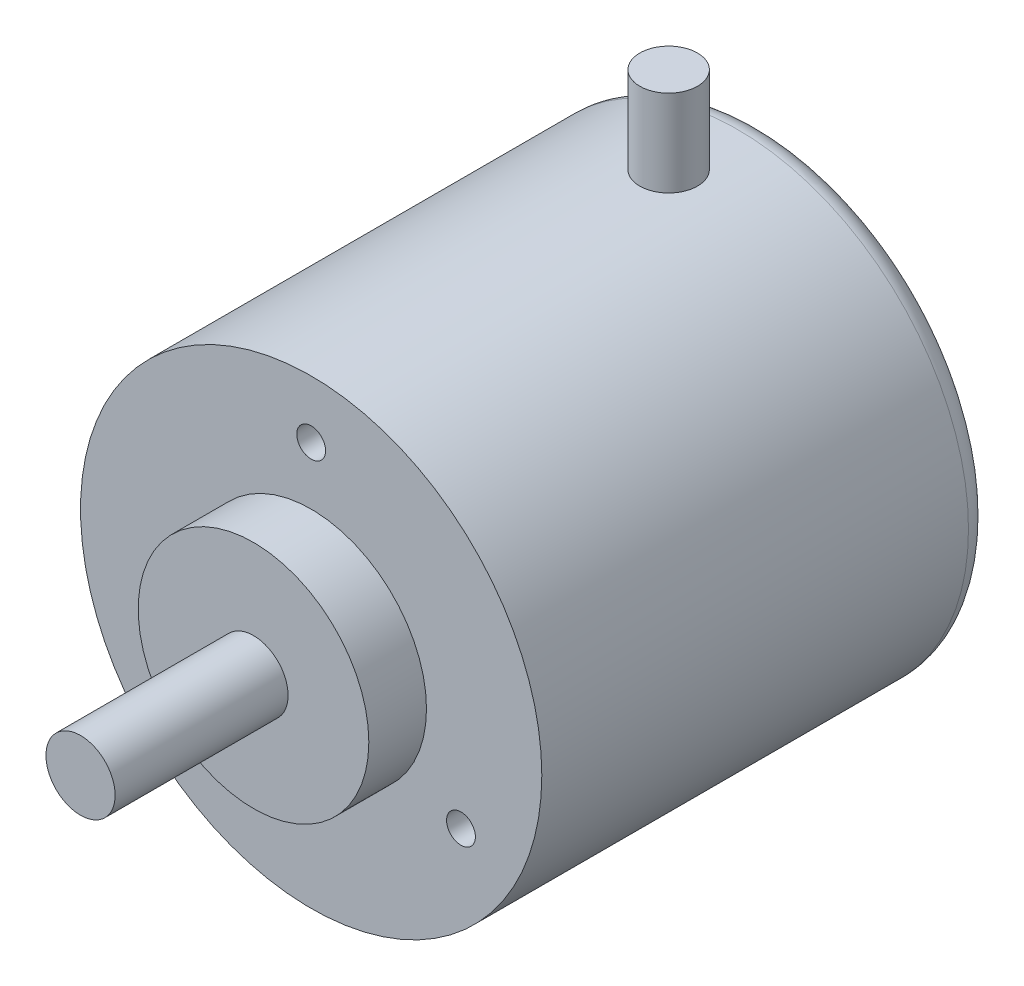
SolidWorks part; units mm, degrees
ref_plane "前视基准面" through (0, 0, 0) normal (0, 0, 1) x (1, 0, 0)
ref_plane "上视基准面" through (0, 0, 0) normal (0, 1, 0) x (1, 0, 0)
ref_plane "右视基准面" through (0, 0, 0) normal (1, 0, 0) x (0, 0, -1)
sketch "草图1" plane through (0, 0, 0) normal (0, 0, 1) x (1, 0, 0)
  circle A0 centre (0, 0) radius 20
extrude "凸台-拉伸1" add sketch "草图1" along normal blind 39
sketch "草图2" plane through (0, 0, 39) normal (0, 0, 1) x (1, 0, 0)
  circle A0 centre (0, 0) radius 10
extrude "凸台-拉伸2" add sketch "草图2" along normal blind 5 separate body
sketch "草图3" plane through (0, 0, 44) normal (0, 0, 1) x (1, 0, 0)
  circle A0 centre (0, 0) radius 3
extrude "凸台-拉伸3" add sketch "草图3" along normal blind 15 separate body
sketch "草图4" plane through (0, 0, 39) normal (0, 0, 1) x (1, 0, 0)
  circle A0 centre (0, 0) radius 15 construction
  circle A1 centre (0, 15) radius 1.5 construction
  circle A2 centre (12.9904, -7.5) radius 1.5 construction
  circle A3 centre (-12.9904, -7.5) radius 1.5 construction
  dimension "D1" = 3
hole_wizard "M3 螺纹孔1" positions "草图5" profile "草图6" tap size "M3" standard "GB"
sketch "草图5" plane through (0, 0, 39) normal (0, 0, 1) x (1, 0, 0)
  circle A0 centre (0, 0) radius 15 construction
  point P0 (0, 15)
  point P4 (-12.9904, -7.5)
  point P7 (12.9904, -7.5)
sketch "草图6" plane through (0, 15, 39) normal (1, 0, 0) x (0, -1, 0)
  line L0 (0, 0) -> (0, 7.5)
  line L1 (0, 7.5) -> (1.25, 6.7489)
  line L2 (1.25, 6.7489) -> (1.25, 0)
  line L5 (1.25, 0) -> (0, 0)
  line L10 (0, 7.5) -> (-1.25, 6.7489) construction
  line L11 (0, -6.35) -> (0, 107.95) construction
  dimension "螺纹孔钻头直径" = 2.5
  dimension "螺纹孔钻头深度" = 7.5
  dimension "导头角度" = 118
cosmetic thread "孔螺蚊线1" parameters "D1"=6, "D2"=3
cosmetic thread "孔螺蚊线2" parameters "D1"=6, "D2"=3
cosmetic thread "孔螺蚊线3" parameters "D1"=6, "D2"=3
fillet "圆角1" radius 2 1 edges at (20, 0, 0)
ref_plane "基准面1" through (0, 20, 0) normal (0, 1, 0) x (1, 0, 0)
sketch "草图8" plane through (0, 20, 0) normal (0, 1, 0) x (1, 0, 0)
  circle A0 centre (0, -8) radius 2.5
  dimension "D2" = 5
  dimension "D1" = 8
extrude "凸台-拉伸4" add sketch "草图8" along normal blind 7.5 separate body
